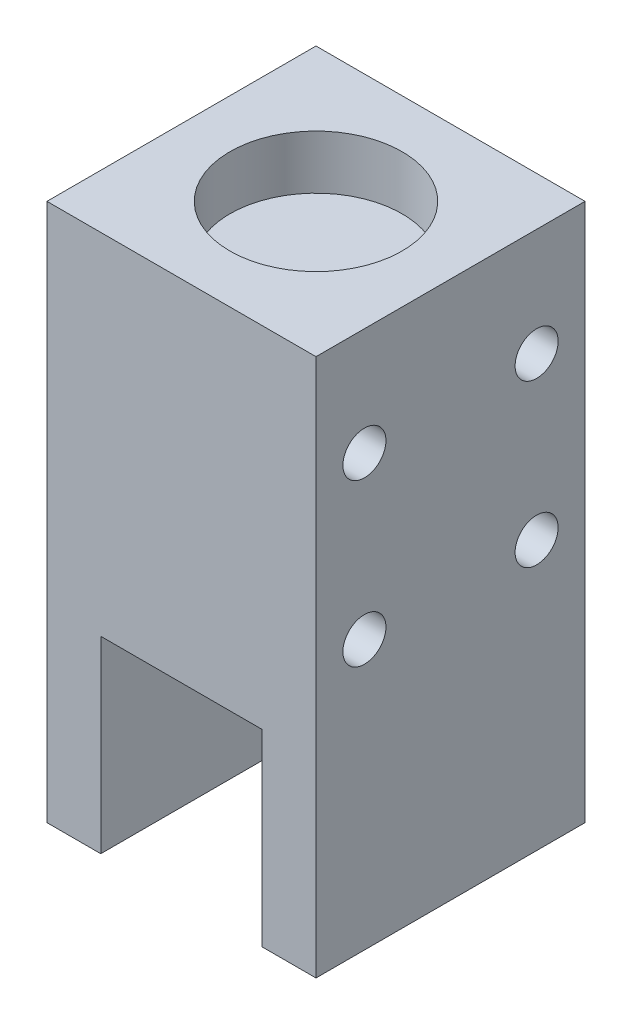
from build123d import *

# Parameters (mm, degrees)
SKETCH1_W           = 50
SKETCH1_H           = 50
BOSS_EXTRUDE1_DEPTH = 100
SKETCH4_W           = 30
SKETCH4_H           = 50
CUT_EXTRUDE2_DEPTH  = 35
SKETCH6_R           = 16
CUT_EXTRUDE3_DEPTH  = 10
SKETCH8_R           = 4
CUT_EXTRUDE6_DEPTH  = 10
CUT_EXTRUDE7_START  = -10
SKETCH9_R           = 4
CUT_EXTRUDE7_DEPTH  = 10


with BuildPart() as part:
    # Sketch1 → Boss-Extrude1 (new body)
    with BuildSketch(Plane(origin=(0, 0, 0), x_dir=(1, 0, 0), z_dir=(0, 1, 0))):
        Rectangle(SKETCH1_W, SKETCH1_H)
    extrude(amount=BOSS_EXTRUDE1_DEPTH)

    # Sketch4 → Cut-Extrude2 (cut)
    with BuildSketch(Plane.XZ):
        Rectangle(SKETCH4_W, SKETCH4_H)
    extrude(amount=-CUT_EXTRUDE2_DEPTH, mode=Mode.SUBTRACT)

    # Sketch6 → Cut-Extrude3 (cut)
    with BuildSketch(Plane(origin=(0, 100, 0), x_dir=(1, 0, 0), z_dir=(0, 1, 0))):
        with Locations(Location((0, 0, 0), (0, 0, 270))):
            Circle(SKETCH6_R)
    extrude(amount=-CUT_EXTRUDE3_DEPTH, mode=Mode.SUBTRACT)

    # Sketch8 → Cut-Extrude6 (cut)
    with BuildSketch(Plane.ZY.offset(25)):
        with Locations((-16, 80)):
            Circle(SKETCH8_R)
        with Locations((16, 80)):
            Circle(SKETCH8_R)
        with Locations((16, 50)):
            Circle(SKETCH8_R)
        with Locations((-16, 50)):
            Circle(SKETCH8_R)
    extrude(amount=-CUT_EXTRUDE6_DEPTH, mode=Mode.SUBTRACT)

    # Sketch9 → Cut-Extrude7 (cut)
    with BuildSketch(Plane(origin=(25, 0, 0), x_dir=(0, 0, -1), z_dir=(1, 0, 0)).offset(CUT_EXTRUDE7_START)):
        with Locations(Location((-16, 80, 0), (0, 0, 180))):
            Circle(SKETCH9_R)
        with Locations(Location((-16, 50, 0), (0, 0, 180))):
            Circle(SKETCH9_R)
        with Locations(Location((16, 50, 0), (0, 0, 180))):
            Circle(SKETCH9_R)
        with Locations(Location((16, 80, 0), (0, 0, 180))):
            Circle(SKETCH9_R)
    extrude(amount=CUT_EXTRUDE7_DEPTH, mode=Mode.SUBTRACT)


solid = part.part
